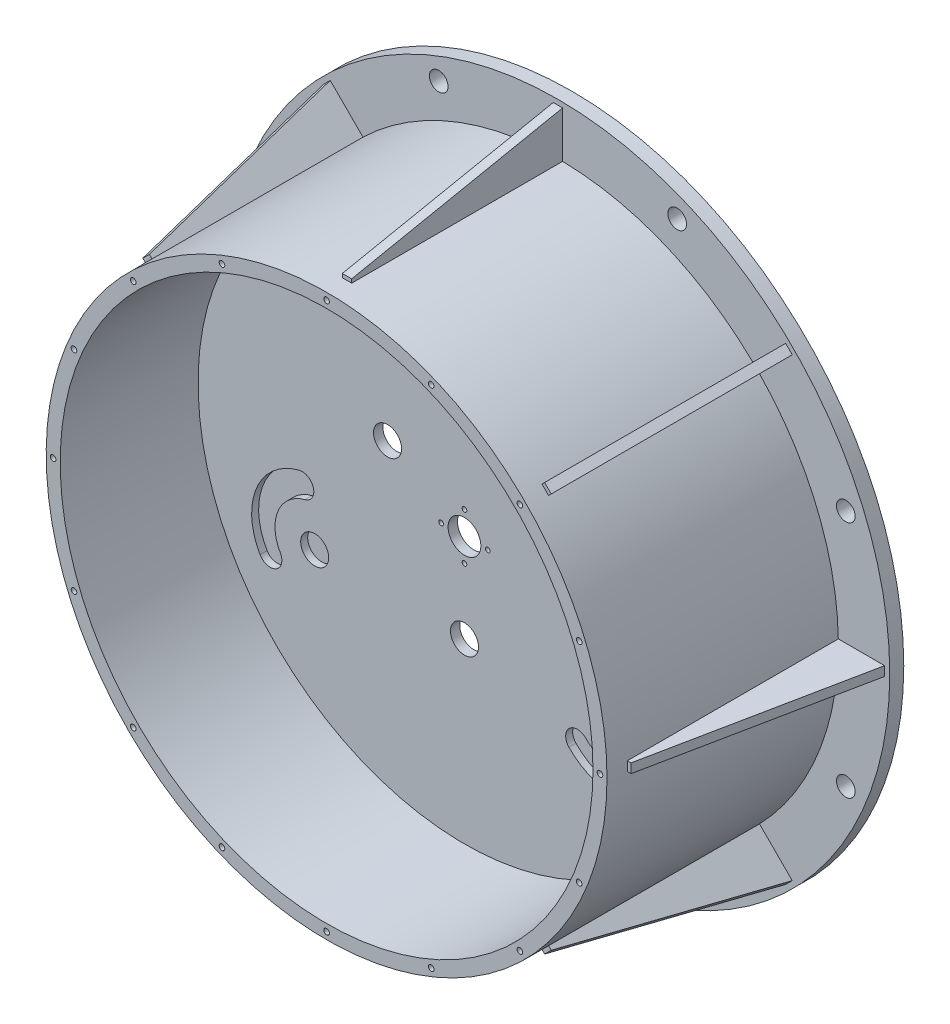
from build123d import *

# Parameters (mm, degrees)
SKETCH1_R           = 600
BOSS_EXTRUDE1_DEPTH = 20
SKETCH2_R           = 35
SKETCH2_R_2         = 5
CUT_EXTRUDE1_DEPTH  = 849.763806957
SKETCH3_R           = 30
CUT_EXTRUDE2_DEPTH  = 849.763806957
CIRPATTERN1_COUNT   = 3
BOSS_EXTRUDE2_START = -200
SKETCH4_R           = 600
SKETCH4_R_2         = 570
BOSS_EXTRUDE2_DEPTH = 200
SKETCH6_R           = 30
CUT_EXTRUDE3_DEPTH  = 15
SKETCH7_R           = 600
SKETCH7_R_2         = 570
BOSS_EXTRUDE3_DEPTH = 295
BOSS_EXTRUDE4_START = 30
SKETCH8_R           = 710
SKETCH8_R_2         = 570
SKETCH8_R_3         = 20
BOSS_EXTRUDE4_DEPTH = 30
SKETCH9_R           = 6
CUT_EXTRUDE4_DEPTH  = 30
BOSS_EXTRUDE5_DEPTH = 10
CIRPATTERN2_COUNT   = 8


with BuildPart() as part:
    # Sketch1 → Boss-Extrude1 (new body)
    with BuildSketch(Plane.XY):
        Circle(SKETCH1_R)
    extrude(amount=BOSS_EXTRUDE1_DEPTH)

    # Sketch2 → Cut-Extrude1 (cut, through all)
    with BuildSketch(Plane(origin=(0, 0, 0), x_dir=(-1, 0, 0), z_dir=(0, 0, -1))):
        Circle(SKETCH2_R)
        with Locations((50, 0)):
            Circle(SKETCH2_R_2)
        with Locations((0, -50)):
            Circle(SKETCH2_R_2)
        with Locations((-50, 0)):
            Circle(SKETCH2_R_2)
        with Locations((0, 50)):
            Circle(SKETCH2_R_2)
    extrude(amount=-CUT_EXTRUDE1_DEPTH, mode=Mode.SUBTRACT)

    # Sketch3 → Cut-Extrude2 (cut, through all)
    with BuildSketch(Plane(origin=(0, 0, 0), x_dir=(-1, 0, 0), z_dir=(0, 0, -1))):
        with Locations((0, -190)):
            Circle(SKETCH3_R)
    cut_extrude2 = extrude(amount=-CUT_EXTRUDE2_DEPTH, mode=Mode.SUBTRACT)

    # CirPattern1: Cut-Extrude2 ×3 about axis
    cirpattern1_axis = Axis((0, 0, 0), (0, 0, 1))
    for i in range(1, CIRPATTERN1_COUNT):
        add(cut_extrude2.rotate(cirpattern1_axis, i * 360 / CIRPATTERN1_COUNT), mode=Mode.SUBTRACT)

    # Sketch4 → Boss-Extrude2 (add)
    with BuildSketch(Plane.XY.offset(20).offset(BOSS_EXTRUDE2_START)):
        Circle(SKETCH4_R)
        Circle(SKETCH4_R_2, mode=Mode.SUBTRACT)
    extrude(amount=BOSS_EXTRUDE2_DEPTH)

    # Sketch6 → Cut-Extrude3 (cut)
    with BuildSketch(Plane.XY.offset(20)):
        with Locations((0, 370)):
            Circle(SKETCH6_R)
        with Locations((320.4293994, -185)):
            Circle(SKETCH6_R)
        with Locations((-320.4293994, -185)):
            Circle(SKETCH6_R)
        with BuildLine():
            ThreePointArc((437.342828911, -252.5), (428.192193817, -218.349364905), (394.041558722, -227.5))
            ThreePointArc((394.041558722, -227.5), (330.915930172, -269.350653064), (259.464472051, -244.230715286))
            ThreePointArc((259.464472051, -244.230715286), (224.112812452, -243.720652914), (223.60275008, -279.072312513))
            ThreePointArc((223.60275008, -279.072312513), (337.084477685, -318.968684279), (437.342828911, -252.5))
        make_face()
        with BuildLine():
            ThreePointArc((-437.342828911, -252.5), (-403.192193817, -261.650635095), (-394.041558722, -227.5))
            ThreePointArc((-394.041558722, -227.5), (-398.722473166, -151.906275514), (-341.242239847, -102.587466532))
            ThreePointArc((-341.242239847, -102.587466532), (-323.124683076, -72.22706244), (-353.485087169, -54.109505669))
            ThreePointArc((-353.485087169, -54.109505669), (-444.777222439, -132.439378757), (-437.342828911, -252.5))
        make_face()
        with BuildLine():
            ThreePointArc((81.777767797, 346.818181818), (67.806542993, 421.256928578), (0, 455))
            ThreePointArc((0, 455), (-25, 480), (0, 505))
            ThreePointArc((0, 505), (107.692744754, 451.408063036), (129.882337089, 333.181818182))
            ThreePointArc((129.882337089, 333.181818182), (99.011870624, 315.947715354), (81.777767797, 346.818181818))
        make_face()
    extrude(amount=-CUT_EXTRUDE3_DEPTH, mode=Mode.SUBTRACT)

    # Sketch7 → Boss-Extrude3 (add)
    with BuildSketch(Plane.XY.offset(20)):
        Circle(SKETCH7_R)
        Circle(SKETCH7_R_2, mode=Mode.SUBTRACT)
    extrude(amount=BOSS_EXTRUDE3_DEPTH)

    # Sketch8 → Boss-Extrude4 (add)
    with BuildSketch(Plane(origin=(0, 0, -180), x_dir=(-1, 0, 0), z_dir=(0, 0, -1)).offset(BOSS_EXTRUDE4_START)):
        Circle(SKETCH8_R)
        with Locations(Location((0, 0, 0), (0, 0, 180))):
            Circle(SKETCH8_R_2, mode=Mode.SUBTRACT)
        with Locations((-615.980281024, 255.147386555)):
            Circle(SKETCH8_R_3, mode=Mode.SUBTRACT)
        with Locations((-255.147386555, 615.980281024)):
            Circle(SKETCH8_R_3, mode=Mode.SUBTRACT)
        with Locations((255.147386555, 615.980281024)):
            Circle(SKETCH8_R_3, mode=Mode.SUBTRACT)
        with Locations((615.980281024, 255.147386555)):
            Circle(SKETCH8_R_3, mode=Mode.SUBTRACT)
        with Locations((615.980281024, -255.147386555)):
            Circle(SKETCH8_R_3, mode=Mode.SUBTRACT)
        with Locations((255.147386555, -615.980281024)):
            Circle(SKETCH8_R_3, mode=Mode.SUBTRACT)
        with Locations((-255.147386555, -615.980281024)):
            Circle(SKETCH8_R_3, mode=Mode.SUBTRACT)
        with Locations((-615.980281024, -255.147386555)):
            Circle(SKETCH8_R_3, mode=Mode.SUBTRACT)
    extrude(amount=-BOSS_EXTRUDE4_DEPTH)

    # Sketch9 → Cut-Extrude4 (cut)
    with BuildSketch(Plane.XY.offset(315)):
        with Locations((585, 0)):
            Circle(SKETCH9_R)
        with Locations((540.469526519, -223.869807934)):
            Circle(SKETCH9_R)
        with Locations((413.657466994, -413.657466994)):
            Circle(SKETCH9_R)
        with Locations((223.869807934, -540.469526519)):
            Circle(SKETCH9_R)
        with Locations((0, -585)):
            Circle(SKETCH9_R)
        with Locations((-223.869807934, -540.469526519)):
            Circle(SKETCH9_R)
        with Locations((-413.657466994, -413.657466994)):
            Circle(SKETCH9_R)
        with Locations((-540.469526519, -223.869807934)):
            Circle(SKETCH9_R)
        with Locations((-585, 0)):
            Circle(SKETCH9_R)
        with Locations((-540.469526519, 223.869807934)):
            Circle(SKETCH9_R)
        with Locations((-413.657466994, 413.657466994)):
            Circle(SKETCH9_R)
        with Locations((-223.869807934, 540.469526519)):
            Circle(SKETCH9_R)
        with Locations((0, 585)):
            Circle(SKETCH9_R)
        with Locations((223.869807934, 540.469526519)):
            Circle(SKETCH9_R)
        with Locations((413.657466994, 413.657466994)):
            Circle(SKETCH9_R)
        with Locations((540.469526519, 223.869807934)):
            Circle(SKETCH9_R)
    extrude(amount=-CUT_EXTRUDE4_DEPTH, mode=Mode.SUBTRACT)

    # Sketch10 → Boss-Extrude5 (add, symmetric)
    with BuildSketch(Plane(origin=(0, 0, 0), x_dir=(1, 0, 0), z_dir=(0, 1, 0))):
        Polygon((-594.317613538, 180), (-594.317613538, -271.329587104), (-607.936057575, -271.329587104), (-698.993694982, 180), align=None)
    boss_extrude5 = extrude(amount=BOSS_EXTRUDE5_DEPTH, both=True)

    # CirPattern2: Boss-Extrude5 ×8 about axis
    cirpattern2_axis = Axis((0, 0, 0), (0, 0, 1))
    for i in range(1, CIRPATTERN2_COUNT):
        add(boss_extrude5.rotate(cirpattern2_axis, i * 360 / CIRPATTERN2_COUNT))


solid = part.part
